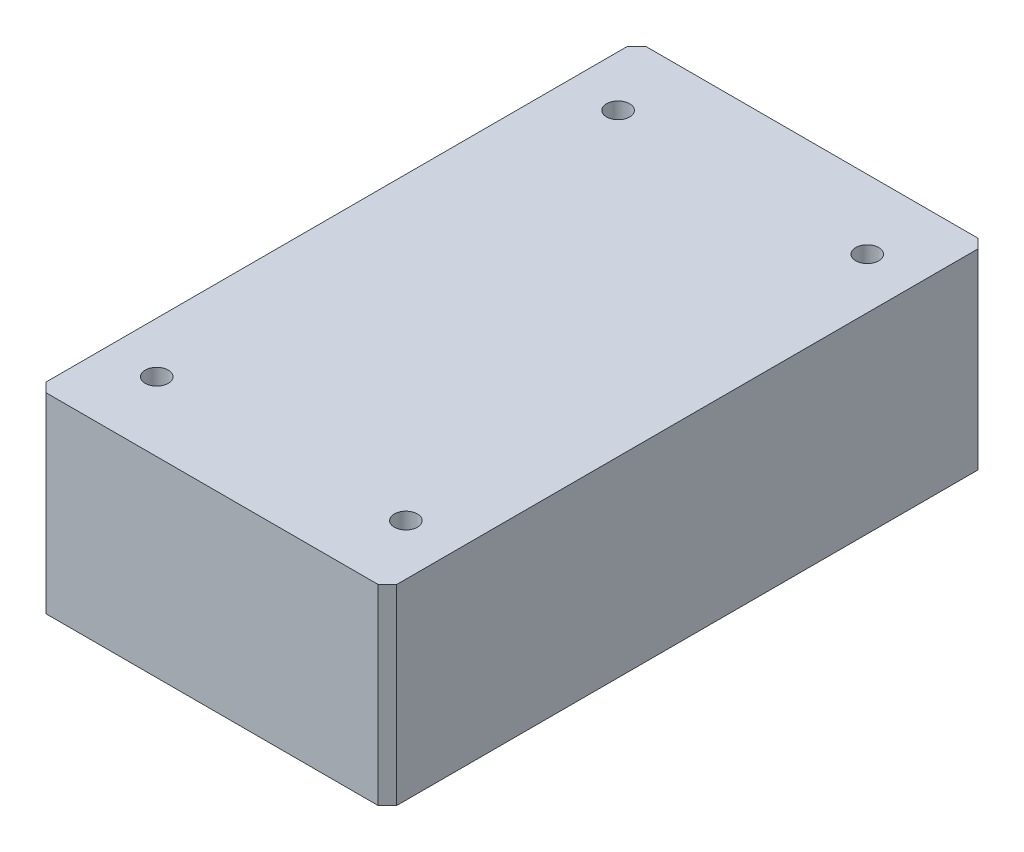
from build123d import *

# Parameters (mm, degrees)
SKETCH_1_W         = 76
SKETCH_1_H         = 41.5
EXTRUDE_1_DEPTH    = 65
HOLE_WIZARD_M6_1_D = 5
CHAMFER_1_SIZE     = 2


with BuildPart() as part:
    # 草图1 → 凸台-拉伸1 (new, symmetric)
    with BuildSketch(Plane.XY):
        Rectangle(SKETCH_1_W, SKETCH_1_H)
    extrude(amount=EXTRUDE_1_DEPTH, both=True)

    # M6 螺纹孔1 (through all)
    with Locations(Plane(origin=(0, 20.75, 0), x_dir=(1, 0, 0), z_dir=(0, 1, 0))):
        with Locations((-27.000001035, -50), (27.000001035, -50), (27.000001035, 50), (-27.000001035, 50)):
            Hole(HOLE_WIZARD_M6_1_D / 2)

    # 倒角1
    chamfer_1_edges = [part.edges().sort_by_distance(p)[0] for p in [
        (-38, 0, 65),
        (38, 0, 65),
        (-38, 0, -65),
        (38, 0, -65),
    ]]
    chamfer(chamfer_1_edges, length=CHAMFER_1_SIZE)


solid = part.part
